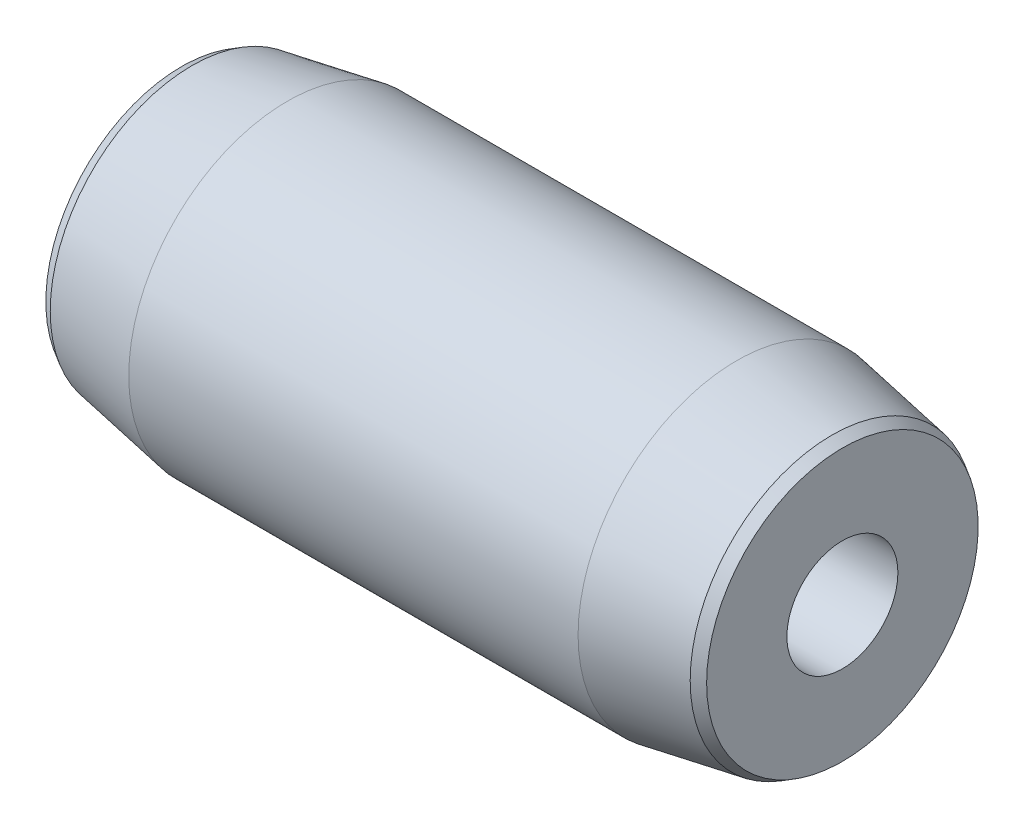
SolidWorks part; units mm, degrees
material "42CrMo"
ref_plane "前视基准面" through (0, 0, 0) normal (0, 0, 1) x (1, 0, 0)
ref_plane "上视基准面" through (0, 0, 0) normal (0, 1, 0) x (1, 0, 0)
ref_plane "右视基准面" through (0, 0, 0) normal (1, 0, 0) x (0, 0, -1)
sketch "草图1" plane through (0, 0, 0) normal (0, 0, 1) x (1, 0, 0)
  line L0 (0, 0) -> (81.9641, 0) construction
  line L1 (0, 0) -> (0, 26.4735)
  line L2 (0, 26.4735) -> (20, 30)
  line L3 (20, 30) -> (105, 30)
  line L4 (62.5, 0) -> (62.5, 30) construction
  line L5 (125, 26.4735) -> (105, 30)
  line L6 (125, 0) -> (125, 26.4735)
  line L7 (0, 0) -> (125, 0)
  dimension "D1" = 30
  dimension "D2" = 10
  dimension "D3" = 20
  dimension "D4" = 125
revolve "旋转1" add sketch "草图1" angle 360 about L7
sketch "草图2" plane through (125, 0, 0) normal (1, 0, 0) x (0, 0, -1)
  circle A0 centre (0, 0) radius 10.5
  dimension "D1" = 21
extrude "切除-拉伸1" cut sketch "草图2" against normal through all
hole_wizard "M24 螺纹孔2" positions "3D草图2" profile "草图4" tap size "M24" standard "GB"
sketch3d "3D草图2"
  circle A0 centre (0, 0, 0) radius 26.4735 construction
  point P0 (0, 0, 0)
  point P5 (-26.4735, 0, 0)
sketch "草图4" plane through (0, 0, 0) normal (0, 1, 0) x (0, 0, 1)
  line L0 (0, 0) -> (0, 69.309)
  line L1 (0, 69.309) -> (10.5, 63)
  line L2 (10.5, 63) -> (10.5, 0)
  line L5 (10.5, 0) -> (0, 0)
  line L10 (0, 69.309) -> (-10.5, 63) construction
  line L11 (0, -6.35) -> (0, 107.95) construction
  dimension "螺纹孔钻头直径" = 21
  dimension "螺纹孔钻头深度" = 63
  dimension "导头角度" = 118
cosmetic thread "孔螺蚊线1" parameters "D1"=48, "D2"=24
chamfer "倒角1" distance 2 angle 20 2 edges at (0, 0, 26.4735) (125, 0, 26.4735)
